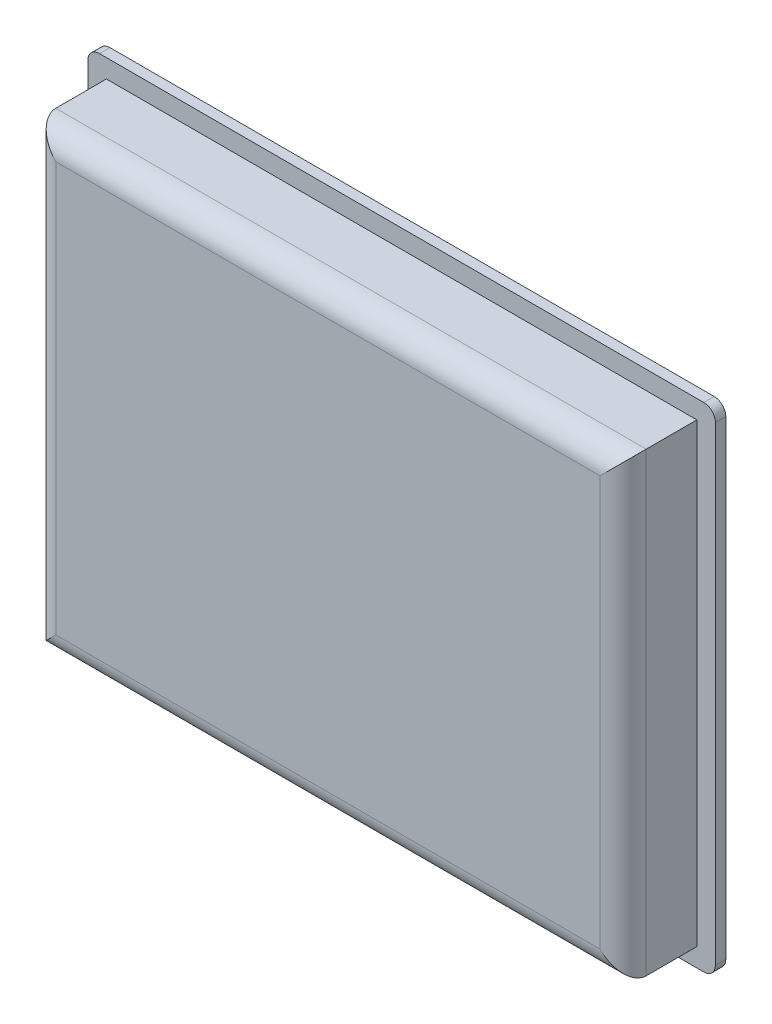
SolidWorks part; units mm, degrees
ref_plane "前视" through (0, 0, 0) normal (0, 0, 1) x (1, 0, 0)
ref_plane "上视" through (0, 0, 0) normal (0, 1, 0) x (1, 0, 0)
ref_plane "右视" through (0, 0, 0) normal (1, 0, 0) x (0, 0, -1)
sketch "草图1" plane through (0, 0, 0) normal (0, 0, 1) x (1, 0, 0)
  line L1 (0, 0) -> (271, 0)
  line L2 (0, 0) -> (0, -213)
  line L3 (0, -213) -> (271, -213)
  line L4 (271, 0) -> (271, -213)
  dimension "D1" = 271
  dimension "D2" = 213
extrude "凸台-拉伸1" add sketch "草图1" along normal blind 4.5
sketch "草图2" plane through (0, 0, 4.5) normal (0, 0, 1) x (1, 0, 0)
  line L0 (135.5, 0) -> (135.5, -213) construction
  line L1 (271, 0) -> (0, 0) construction
  line L2 (0, -213) -> (271, -213) construction
  line L4 (8, -8) -> (263, -8)
  line L5 (8, -8) -> (8, -205)
  line L6 (8, -205) -> (263, -205)
  line L7 (263, -8) -> (263, -205)
  line L8 (8, -8) -> (263, -205) construction
  line L9 (8, -205) -> (263, -8) construction
  point P6 (135.5, -106.5)
  dimension "D1" = 197
  dimension "D2" = 255
extrude "凸台-拉伸2" add sketch "草图2" along normal blind 31.86
fillet "圆角1" radius 10 4 edges at (135.5, -205, 36.36) (8, -106.5, 36.36) (135.5, -8, 36.36) (263, -106.5, 36.36)
fillet "圆角2" radius 5 4 edges at (0, -213, 2.25) (271, -213, 2.25) (271, 0, 2.25) (0, 0, 2.25)
sketch "草图4" plane through (0, 0, 0) normal (0, 0, -1) x (-1, 0, 0)
  line L0 (-271, -106.5) -> (0, -106.5) construction
  line L1 (-271, -208) -> (-271, -5) construction
  line L2 (0, -5) -> (0, -208) construction
  line L4 (-245.5, -36.5) -> (-25.5, -36.5)
  line L5 (-245.5, -36.5) -> (-245.5, -176.5)
  line L6 (-245.5, -176.5) -> (-25.5, -176.5)
  line L7 (-25.5, -36.5) -> (-25.5, -176.5)
  line L8 (-245.5, -36.5) -> (-25.5, -176.5) construction
  line L9 (-245.5, -176.5) -> (-25.5, -36.5) construction
  point P6 (-135.5, -106.5)
  dimension "D1" = 140
  dimension "D2" = 220
extrude "切除-拉伸1" cut sketch "草图4" against normal blind 3
